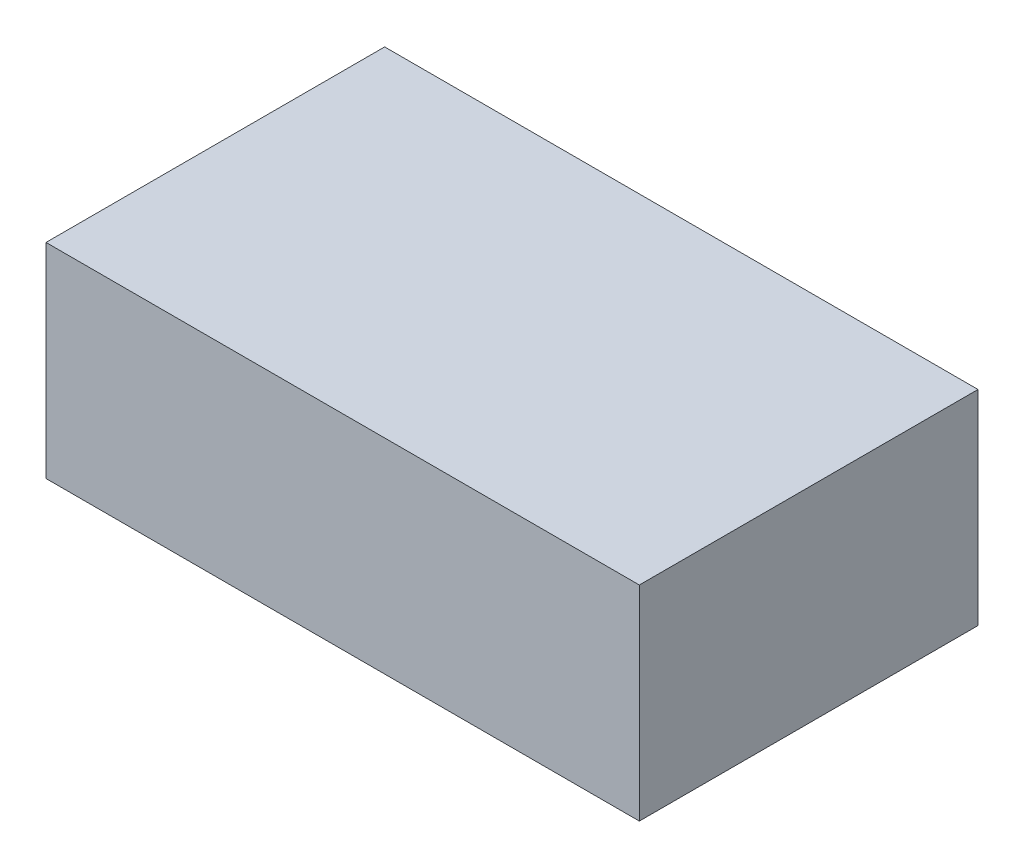
SolidWorks part; units mm, degrees
ref_plane "前视基准面" through (0, 0, 0) normal (0, 0, 1) x (1, 0, 0)
ref_plane "上视基准面" through (0, 0, 0) normal (0, 1, 0) x (1, 0, 0)
ref_plane "右视基准面" through (0, 0, 0) normal (1, 0, 0) x (0, 0, -1)
sketch "草图1" plane through (0, 0, 0) normal (0, 1, 0) x (1, 0, 0)
  line L1 (-3250, 1855) -> (3250, 1855)
  line L2 (-3250, 1855) -> (-3250, -1855)
  line L3 (-3250, -1855) -> (3250, -1855)
  line L4 (3250, 1855) -> (3250, -1855)
  line L5 (-3250, 1855) -> (3250, -1855) construction
  line L6 (-3250, -1855) -> (3250, 1855) construction
  point P0 (0, 0)
  dimension "D1" = 6500
  dimension "D2" = 3710
extrude "凸台-拉伸1" add sketch "草图1" along normal blind 2240
sketch "草图2" plane through (0, 0, 0) normal (1, 0, 0) x (0, 0, -1)
  line L0 (0, 2240) -> (0, 0) construction
  line L1 (-1855, 2240) -> (1855, 2240) construction
  line L3 (-1825, 30) -> (1825, 30)
  line L4 (-1825, 30) -> (-1825, 2210)
  line L5 (-1825, 2210) -> (1825, 2210)
  line L6 (1825, 30) -> (1825, 2210)
  line L7 (-1825, 30) -> (1825, 2210) construction
  line L8 (-1825, 2210) -> (1825, 30) construction
  point P5 (0, 1120)
  dimension "D1" = 3650
  dimension "D2" = 2180
extrude "切除-拉伸1" cut sketch "草图2" against normal blind 3220 and the other way blind 3220
